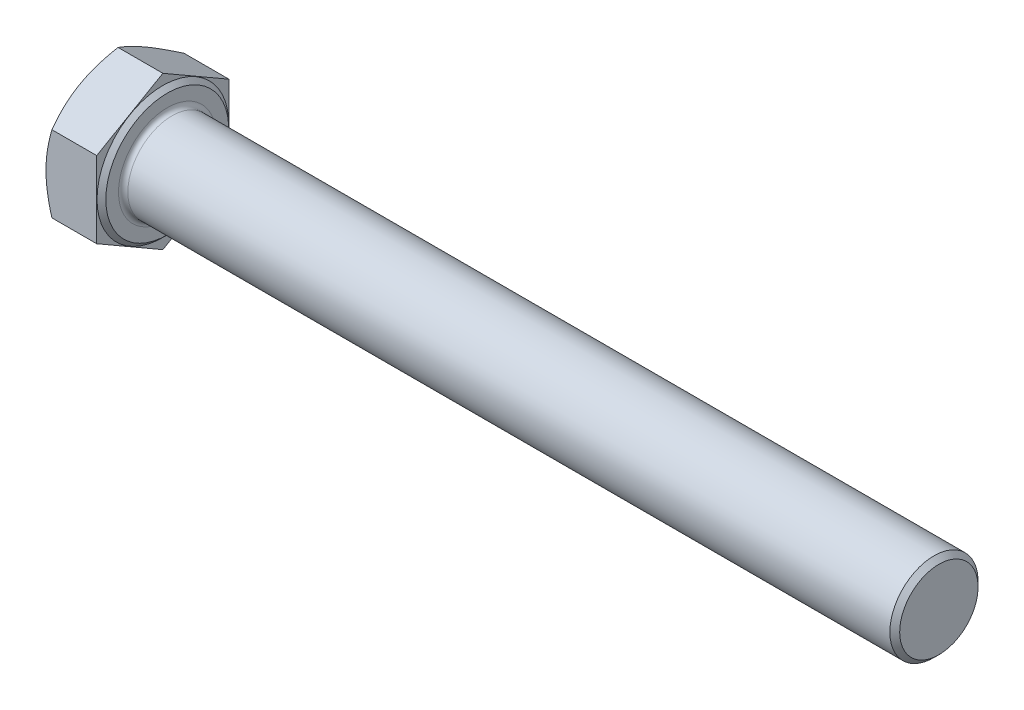
SolidWorks part; units mm, degrees
material "Q235"
ref_plane "Front Plane" through (0, 0, 0) normal (0, 0, 1) x (1, 0, 0)
ref_plane "Top Plane" through (0, 0, 0) normal (0, 1, 0) x (1, 0, 0)
ref_plane "Right Plane" through (0, 0, 0) normal (1, 0, 0) x (0, 0, -1)
sketch "Sketch1" plane through (0, 0, 0) normal (0, 0, 1) x (1, 0, 0)
  line L0 (0, 0) -> (150, 0) construction
  line L1 (0, 0) -> (0, 13.375)
  line L2 (0, 13.375) -> (10, 13.375)
  line L3 (10, 13.375) -> (10, 0)
  line L4 (10, 8) -> (150, 8)
  line L5 (150, 8) -> (150, 0)
  line L6 (0, 12) -> (0.7939, 13.375)
  line L7 (146, 8) -> (146, 0)
  line L8 (16, 8) -> (16, 0)
  line L9 (10, 7.3505) -> (150, 7.3505)
  line L10 (150, 6.9175) -> (10, 6.9175)
  line L11 (9.2, 11.945) -> (10, 11.145)
  line L12 (9.2, 13.375) -> (9.2, 0)
  line L13 (9.9, 11.245) -> (9.9, 0) construction
  arc A0 (10, 8.85) -> (10.85, 8) centre (10.85, 8.85) ccw
  point P12 (148, 0)
  point P13 (3.13, 13.375)
  point P14 (10, 8.85)
  point P24 (10, 11.245)
  dimension "D1" = 0.1
  dimension "r" = 0.85
  dimension "k" = 10
  dimension "D2" = 45
  dimension "β" = 30
  dimension "e" = 26.75
  dimension "s" = 24
  dimension "d" = 16
  dimension "l" = 140
  dimension "D52" = 4
  dimension "P" = 2
  dimension "kw" = 6.87
  dimension "da" = 17.7
  dimension "a" = 6
  dimension "ds" = 14.701
  dimension "D61" = 13.835
  dimension "dw" = 22.49
  dimension "c" = 0.8
sketch "Sketch2" plane through (0, 0, 0) normal (1, 0, 0) x (0, 0, -1)
  line L1 (0, 13.8564) -> (-12, 6.9282)
  line L2 (-12, 6.9282) -> (-12, -6.9282)
  line L3 (-12, -6.9282) -> (0, -13.8564)
  line L4 (0, -13.8564) -> (12, -6.9282)
  line L5 (12, -6.9282) -> (12, 6.9282)
  line L6 (12, 6.9282) -> (0, 13.8564)
  circle A0 centre (0, 0) radius 12 construction
sketch "Sketch3" plane through (0, 0, 0) normal (1, 0, 0) x (0, 0, -1)
  line L0 (12, 6.9282) -> (0, 13.8564) construction
  line L1 (0, 13.8564) -> (-12, 6.9282) construction
  line L2 (-12, 6.9282) -> (-12, -6.9282) construction
  line L3 (12, -6.9282) -> (12, 6.9282) construction
  line L4 (0, -13.8564) -> (12, -6.9282) construction
  line L5 (-12, -6.9282) -> (0, -13.8564) construction
  line L6 (12, 6.9282) -> (0, 13.8564)
  line L7 (0, 13.8564) -> (-12, 6.9282)
  line L8 (-12, 6.9282) -> (-12, -6.9282)
  line L9 (12, -6.9282) -> (12, 6.9282)
  line L10 (0, -13.8564) -> (12, -6.9282)
  line L11 (-12, -6.9282) -> (0, -13.8564)
extrude "Boss-Extrude1" add sketch "Sketch3" along normal up to vertex (10 mm away) up to point (10, 13.375, 0)
sketch "Sketch4" plane through (0, 0, 0) normal (-1, 0, 0) x (0, 0, 1)
  circle A0 centre (0, 0) radius 12 construction
  circle A1 centre (0, 0) radius 12
  circle A2 centre (0, 0) radius 26.75
  dimension "D1" = 53.5
extrude "Cut-Extrude1" cut sketch "Sketch4" against normal blind 1.25 draft 60
sketch "Sketch5" plane through (0, 0, 0) normal (0, 0, 1) x (1, 0, 0)
  line L0 (10, 8) -> (150, 8) construction
  line L1 (150, 8) -> (150, 0) construction
  line L2 (0, 0) -> (150, 0) construction
  line L3 (10.85, 8) -> (150, 8)
  line L4 (150, 8) -> (150, 0)
  line L5 (10, 0) -> (150, 0)
  line L6 (10, 8.85) -> (10, 0)
  arc A0 (10, 8.85) -> (10.85, 8) centre (10.85, 8.85) ccw construction
  arc A1 (10, 8.85) -> (10.85, 8) centre (10.85, 8.85) ccw
revolve "Revolve1" add sketch "Sketch5" angle 360 about L5
cosmetic thread "Cosmetic Thread2" parameters "D1"=64, "D2"=13.835
chamfer "Chamfer2" distance 0.8889 angle 45 1 edges at (150, 0, 8)
sketch "Sketch7" plane through (0, 0, 0) normal (0, 0, 1) x (1, 0, 0)
  line L0 (10, 11.145) -> (9.2, 11.945)
  line L1 (9.2, 11.945) -> (9.2, 26.75)
  line L2 (9.2, 26.75) -> (10, 26.75)
  line L3 (10, 26.75) -> (10, 11.145)
  line L4 (0, 0) -> (150, 0) construction
  line L5 (0, 0) -> (150, 0) construction
  dimension "D1" = 53.5
revolve "Cut-Revolve1" cut sketch "Sketch7" angle 360 mid plane about L5
sketch "Sketch6" [suppressed] plane through (0, 0, 0) normal (0, 0, 1) x (1, 0, 0)
  line L0 (9.3, 0) -> (9.3, 4) construction
  line L1 (9.3, 4) -> (75.3, 4)
  line L2 (75.3, 4) -> (75.3, 0)
  line L3 (9.3, 4) -> (5.9719, 3.5984)
  line L5 (5.3, 3.5941) -> (75.3, 3.5941) construction
  line L6 (5.3, 7.19) -> (5.3, 0) construction
  line L7 (5.3, 4.1941) -> (5.3, 0)
  line L8 (5.3, 0) -> (75.3, 0)
  arc A0 (5.9719, 3.5984) -> (5.3, 4.1941) centre (5.9, 4.1941) cw
  arc A1 (5.3, 4.6) -> (5.9, 4) centre (5.9, 4.6) ccw construction
revolve "Revolve2" add sketch "Sketch6" angle 360 about L8
cosmetic thread "Cosmetic Thread1" [suppressed] parameters "D1"=44, "D2"=13.835
chamfer "Chamfer1" [suppressed] distance 0.8889 angle 45
sketch "Sketch8" [suppressed] plane through (0, 0, 0) normal (0, 0, 1) x (1, 0, 0)
  line L0 (5.3, 5.715) -> (4.7, 6.315)
  line L1 (4.7, 6.315) -> (4.7, 14.38)
  line L2 (4.7, 14.38) -> (5.3, 14.38)
  line L3 (5.3, 14.38) -> (5.3, 5.715)
  line L4 (0, 0) -> (75.3, 0) construction
  line L5 (0, 0) -> (75.3, 0) construction
  dimension "D1" = 53.5
revolve "Cut-Revolve2" [suppressed] cut sketch "Sketch8" angle 360 mid plane about L5
